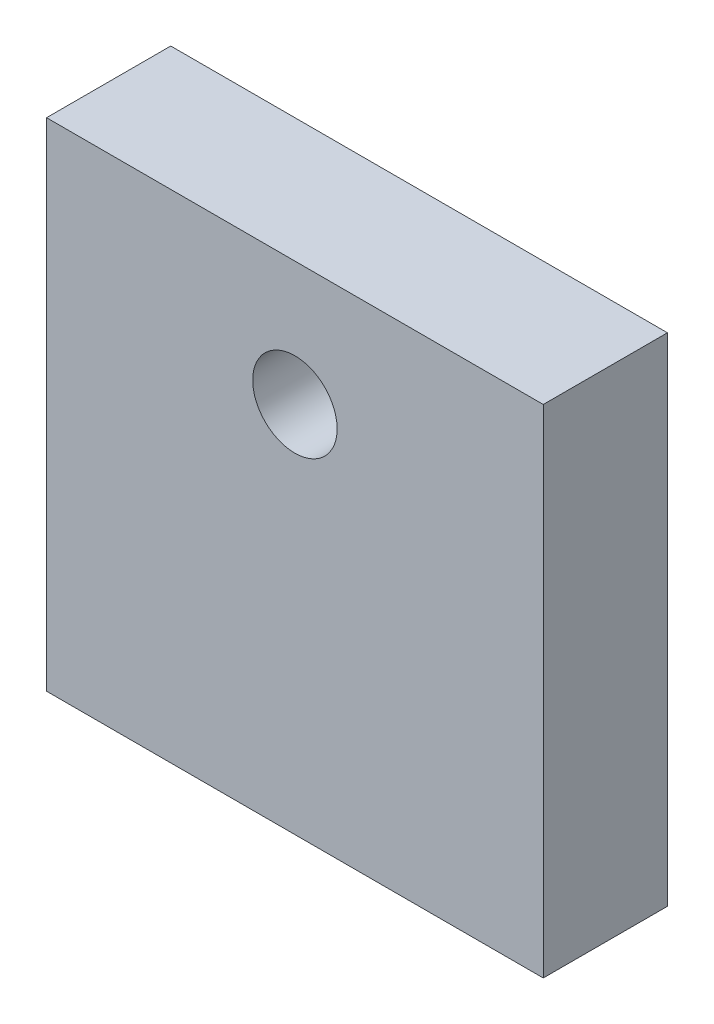
SolidWorks part; units mm, degrees
ref_plane "前视基准面" through (0, 0, 0) normal (0, 0, 1) x (1, 0, 0)
ref_plane "上视基准面" through (0, 0, 0) normal (0, 1, 0) x (1, 0, 0)
ref_plane "右视基准面" through (0, 0, 0) normal (1, 0, 0) x (0, 0, -1)
sketch "草图1" plane through (0, 0, 0) normal (0, 0, 1) x (1, 0, 0)
  line L1 (-20, -20) -> (20, -20)
  line L2 (-20, -20) -> (-20, 20)
  line L3 (-20, 20) -> (20, 20)
  line L4 (20, -20) -> (20, 20)
  line L5 (-20, -20) -> (20, 20) construction
  line L6 (-20, 20) -> (20, -20) construction
  point P0 (0, 0)
  dimension "D1" = 40
  dimension "D2" = 40
extrude "凸台-拉伸1" add sketch "草图1" along normal mid plane 10
hole_wizard "M8 螺纹孔1" positions "草图2" profile "草图3" tap size "M8" standard "GB" end condition through all
sketch "草图2" plane through (0, 0, 5) normal (0, 0, 1) x (1, 0, 0)
  line L0 (-20, 20) -> (-20, -20) construction
  line L1 (-20, -20) -> (20, -20) construction
  point P0 (0, 10)
  dimension "D1" = 20
  dimension "D2" = 30
sketch "草图3" plane through (0, 10, 5) normal (1, 0, 0) x (0, -1, 0)
  line L0 (0, 0) -> (0, 10)
  line L1 (0, 10) -> (3.4, 10)
  line L2 (3.4, 10) -> (3.4, 0)
  line L5 (3.4, 0) -> (0, 0)
  line L11 (0, -6.35) -> (0, 107.95) construction
  dimension "通孔螺纹孔钻头直径" = 6.8
  dimension "通孔螺纹孔钻头深度" = 10
cosmetic thread "孔螺蚊线1"
